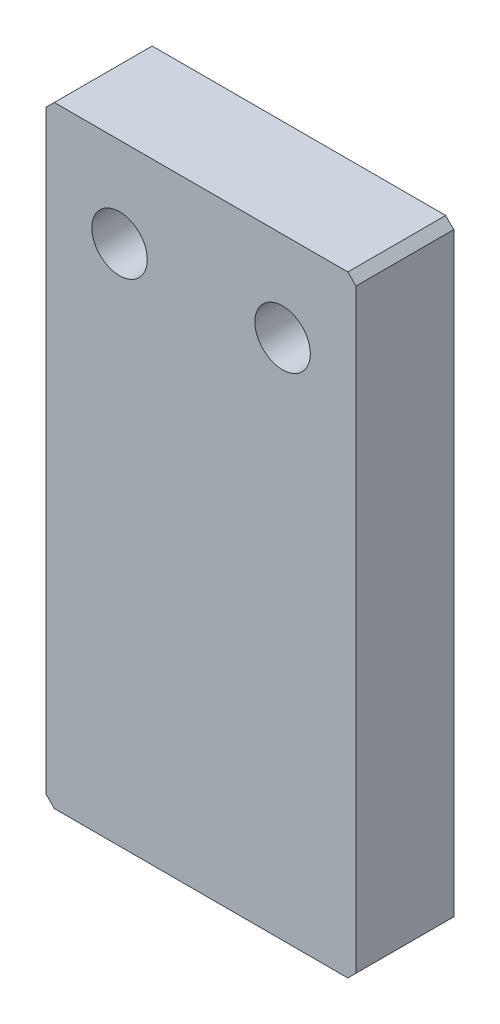
from build123d import *

# Parameters (mm, degrees)
SKETCH1_W             = 38
SKETCH1_H             = 75
BOSS_EXTRUDE1_DEPTH   = 6
M8_TAPPED_HOLE1_D     = 6.8
M8_TAPPED_HOLE2_D     = 6.8
M6_TAPPED_HOLE1_D     = 5
M6_TAPPED_HOLE1_DEPTH = 12
CHAMFER1_SIZE         = 1


with BuildPart() as part:
    # Sketch1 → Boss-Extrude1 (new, symmetric)
    with BuildSketch(Plane.XY):
        Rectangle(SKETCH1_W, SKETCH1_H)
    extrude(amount=BOSS_EXTRUDE1_DEPTH, both=True)

    # M8 Tapped Hole1 (through all)
    with Locations(Plane.XY.offset(6)):
        with Locations((-10, 26.5)):
            Hole(M8_TAPPED_HOLE1_D / 2)

    # M8 Tapped Hole2 (through all)
    with Locations(Plane.XY.offset(6)):
        with Locations((10, 26.5)):
            Hole(M8_TAPPED_HOLE2_D / 2)

    # M6 Tapped Hole1
    with Locations(Plane(origin=(0, -37.5, 0), x_dir=(-1, 0, 0), z_dir=(0, -1, 0))):
        with Locations((10, 0), (-10, 0)):
            Hole(M6_TAPPED_HOLE1_D / 2, depth=M6_TAPPED_HOLE1_DEPTH)

    # Chamfer1
    chamfer1_edges = [part.edges().sort_by_distance(p)[0] for p in [
        (19, -37.5, 0),
        (-19, -37.5, 0),
        (-19, 37.5, 0),
        (19, 37.5, 0),
    ]]
    chamfer(chamfer1_edges, length=CHAMFER1_SIZE)


solid = part.part
